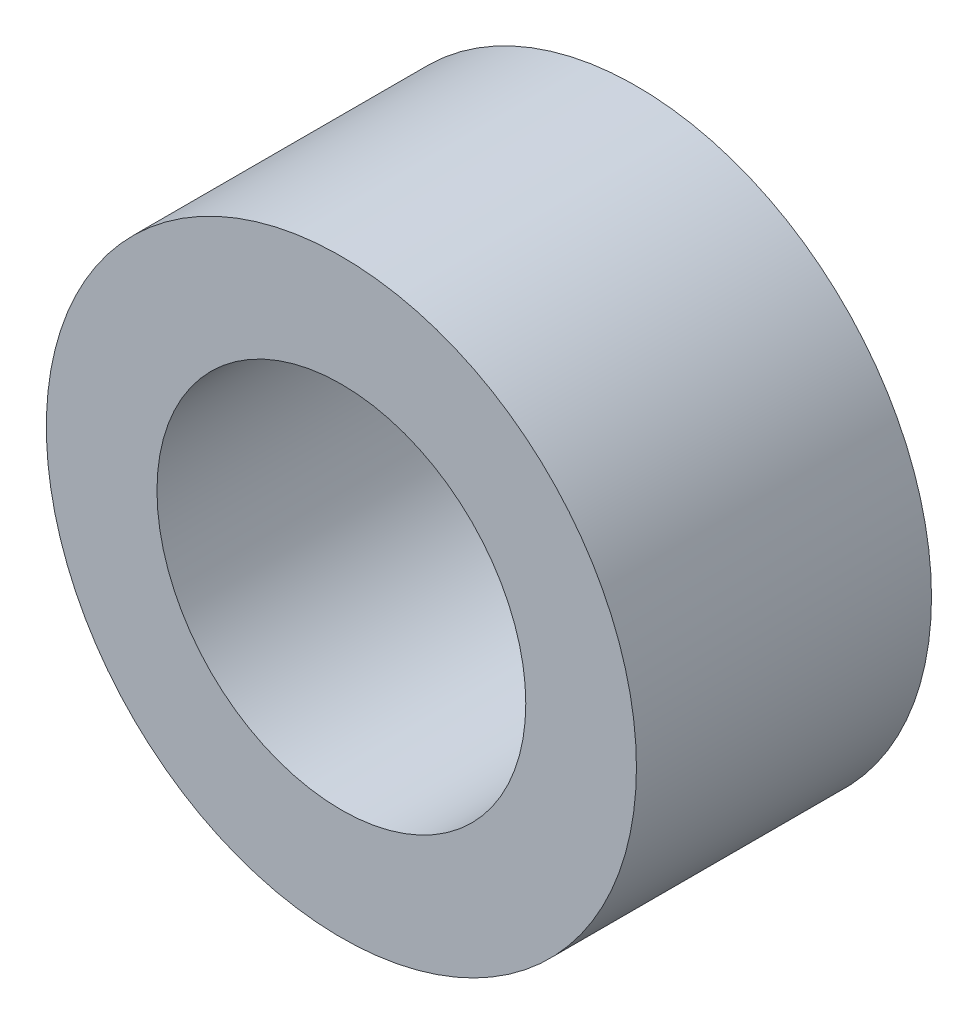
SolidWorks part; units mm, degrees
ref_plane "Front Plane" through (0, 0, 0) normal (0, 0, 1) x (1, 0, 0)
ref_plane "Top Plane" through (0, 0, 0) normal (0, 1, 0) x (1, 0, 0)
ref_plane "Right Plane" through (0, 0, 0) normal (1, 0, 0) x (0, 0, -1)
sketch "Sketch1" plane through (0, 0, 0) normal (0, 0, 1) x (1, 0, 0)
  circle A0 centre (0, 0) radius 5
  circle A1 centre (0, 0) radius 3.125
  dimension "D1" = 10
  dimension "D2" = 6.25
extrude "Boss-Extrude1" add sketch "Sketch1" along normal blind 5
